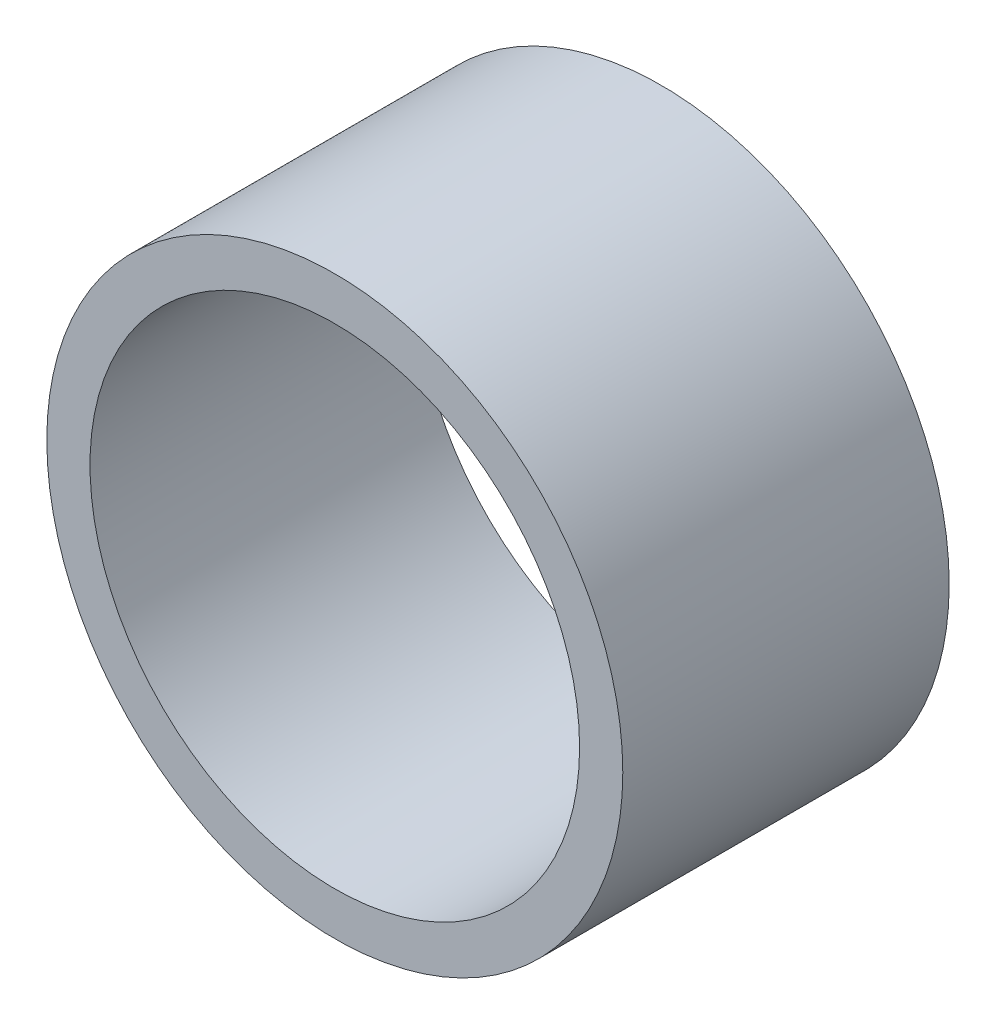
SolidWorks part; units mm, degrees
ref_plane "前视基准面" through (0, 0, 0) normal (0, 0, 1) x (1, 0, 0)
ref_plane "上视基准面" through (0, 0, 0) normal (0, 1, 0) x (1, 0, 0)
ref_plane "右视基准面" through (0, 0, 0) normal (1, 0, 0) x (0, 0, -1)
sketch "草图1" plane through (0, 0, 0) normal (0, 0, 1) x (1, 0, 0)
  circle A0 centre (0, 0) radius 12.75
  circle A1 centre (0, 0) radius 15
  dimension "D1" = 25.5
  dimension "D2" = 30
extrude "凸台-拉伸1" add sketch "草图1" along normal blind 17
